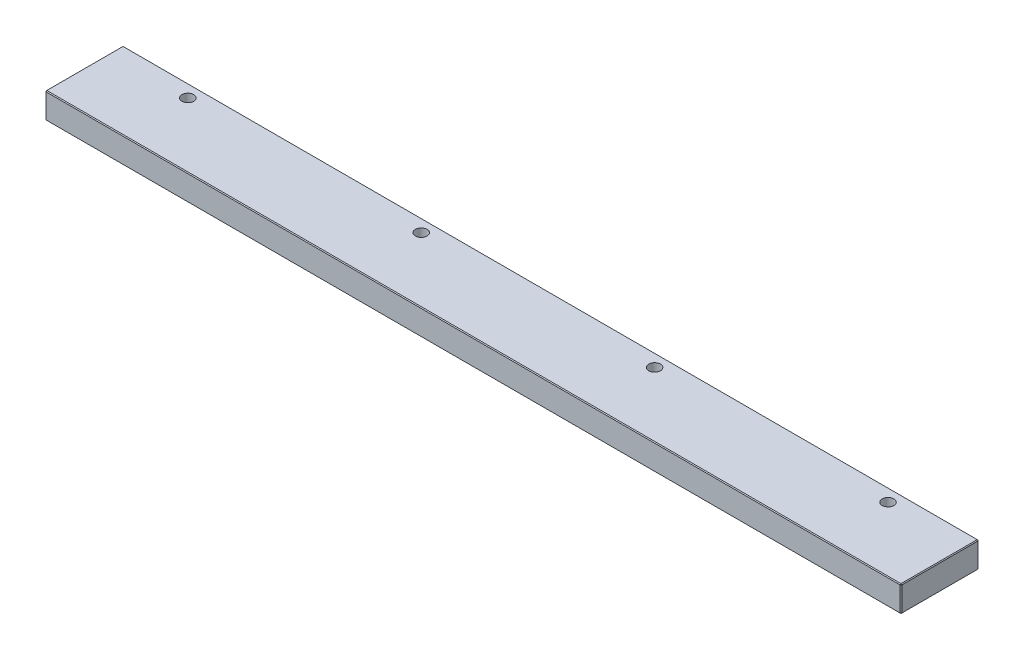
from build123d import *

# Parameters (mm, degrees)
SKETCH_1_W                   = 330
SKETCH_1_H                   = 30
EXTRUDE_1_DEPTH              = 10
HOLE_WIZARD_M4_1_D           = 4.5
HOLE_WIZARD_M4_1_CBORE_D     = 8
HOLE_WIZARD_M4_1_CBORE_DEPTH = 4.4
CHAMFER_1_SIZE               = 0.3


with BuildPart() as part:
    # 草图1 → 凸台-拉伸1 (new body)
    with BuildSketch(Plane(origin=(0, 0, 0), x_dir=(1, 0, 0), z_dir=(0, 1, 0))):
        Rectangle(SKETCH_1_W, SKETCH_1_H)
    extrude(amount=EXTRUDE_1_DEPTH)

    # M4 六角凹头螺钉的柱形沉头孔1 (through all)
    with Locations(Plane(origin=(0, 0, 0), x_dir=(-1, 0, 0), z_dir=(0, -1, 0))):
        with Locations((-135, 10), (-45, 10), (45, 10), (135, 10)):
            CounterBoreHole(HOLE_WIZARD_M4_1_D / 2, HOLE_WIZARD_M4_1_CBORE_D / 2, HOLE_WIZARD_M4_1_CBORE_DEPTH)

    # 倒角1
    chamfer_1_edges = [part.edges().sort_by_distance(p)[0] for p in [
        (-165, 10, 0),
        (0, 10, 15),
        (165, 10, 0),
        (0, 0, 15),
        (-165, 0, 0),
        (0, 0, -15),
        (165, 0, 0),
        (0, 10, -15),
        (165, 5, 15),
        (-165, 5, 15),
        (-165, 5, -15),
        (165, 5, -15),
    ]]
    chamfer(chamfer_1_edges, length=CHAMFER_1_SIZE)


solid = part.part
